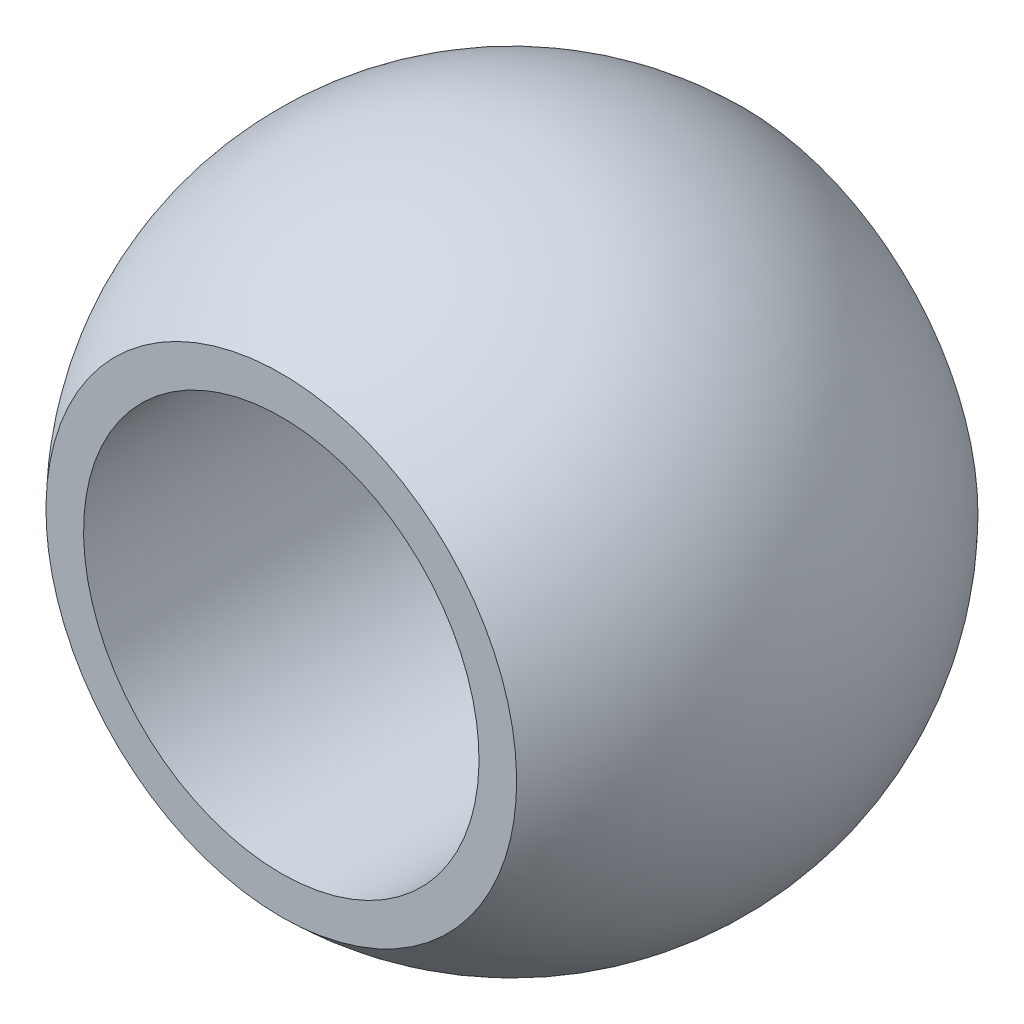
SolidWorks part; units mm, degrees
material "1.0503 (C45)"
ref_plane "前视基准面" through (0, 0, 0) normal (0, 0, 1) x (1, 0, 0)
ref_plane "上视基准面" through (0, 0, 0) normal (0, 1, 0) x (1, 0, 0)
ref_plane "右视基准面" through (0, 0, 0) normal (1, 0, 0) x (0, 0, -1)
sketch "草图1" plane through (0, 0, 0) normal (0, 0, 1) x (1, 0, 0)
  line L0 (0, 50) -> (0, -50)
  arc A0 (0, -50) -> (0, 50) centre (0, 0) ccw
  dimension "D1" = 100
revolve "旋转1" add sketch "草图1" angle 360 about L0
sketch "草图2" plane through (0, 0, 0) normal (0, 0, 1) x (1, 0, 0)
  circle A0 centre (0, 0) radius 30
  dimension "D1" = 60
extrude "切除-拉伸1" cut sketch "草图2" against normal mid plane 100
sketch "草图3" plane through (0, 0, 0) normal (1, 0, 0) x (0, 0, -1)
  line L1 (-35, 60) -> (35, 60)
  line L2 (-35, 60) -> (-35, -60)
  line L3 (-35, -60) -> (35, -60)
  line L4 (35, 60) -> (35, -60)
  line L5 (-35, 60) -> (35, -60) construction
  line L6 (-35, -60) -> (35, 60) construction
  point P0 (0, 0)
  dimension "D1" = 70
  dimension "D2" = 120
extrude "切除-拉伸2" cut sketch "草图3" against normal mid plane 100 flip side to cut
